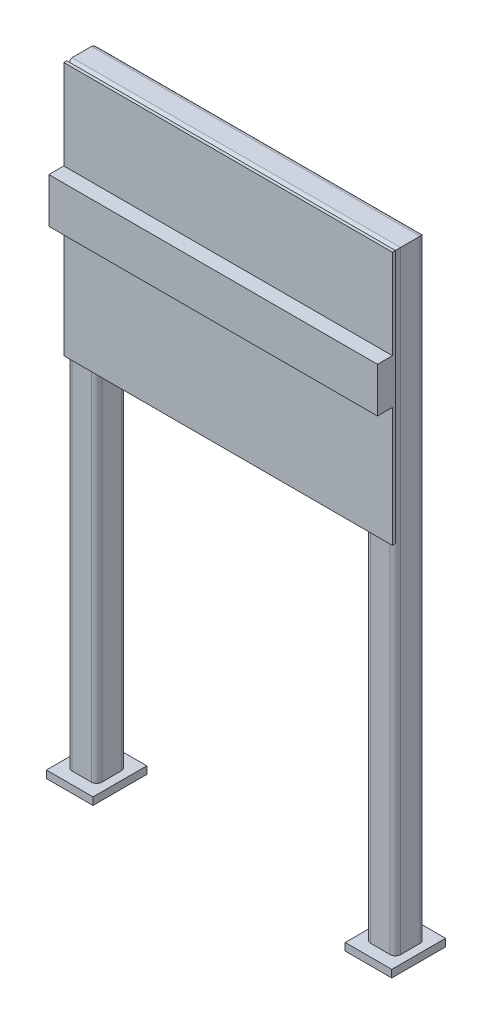
SolidWorks part; units mm, degrees
ref_plane "Front Plane" through (0, 0, 0) normal (0, 0, 1) x (1, 0, 0)
ref_plane "Top Plane" through (0, 0, 0) normal (0, 1, 0) x (1, 0, 0)
ref_plane "Right Plane" through (0, 0, 0) normal (1, 0, 0) x (0, 0, -1)
sketch "草图1" plane through (0, 0, 0) normal (0, 0, 1) x (1, 0, 0)
  line L0 (0, 0) -> (0, 116.4338) construction
  line L1 (-100, 0) -> (-100, 400)
  line L2 (100, 0) -> (100, 400)
  line L3 (-100, 250) -> (100, 250)
  line L4 (-100, 400) -> (100, 400)
  line L5 (-100, 330) -> (100, 330)
  dimension "D1" = 200
  dimension "D2" = 400
  dimension "D3" = 250
  dimension "D4" = 80
other "GB/6728-1986 square hollow section 020 X 20 X 1.75(1)"
ref_plane "Plane1" through (-100, 0, 0) normal (0, 1, 0) x (-1, 0, 0)
sketch "Sketch1" plane through (-100, 0, 0) normal (0, 1, 0) x (-1, 0, 0)
  line L0 (-6.5, -8.25) -> (6.5, -8.25)
  line L1 (-8.25, -6.5) -> (-8.25, 6.5)
  line L2 (6.5, 8.25) -> (-6.5, 8.25)
  line L3 (8.25, 6.5) -> (8.25, -6.5)
  line L4 (-6.5, -10) -> (6.5, -10)
  line L5 (-10, -6.5) -> (-10, 6.5)
  line L6 (6.5, 10) -> (-6.5, 10)
  line L7 (10, 6.5) -> (10, -6.5)
  arc A0 (10, 6.5) -> (6.5, 10) centre (6.5, 6.5) ccw
  arc A1 (6.5, -10) -> (10, -6.5) centre (6.5, -6.5) ccw
  arc A2 (-10, -6.5) -> (-6.5, -10) centre (-6.5, -6.5) ccw
  arc A3 (-6.5, 10) -> (-10, 6.5) centre (-6.5, 6.5) ccw
  arc A4 (-6.5, 8.25) -> (-8.25, 6.5) centre (-6.5, 6.5) ccw
  arc A5 (8.25, 6.5) -> (6.5, 8.25) centre (6.5, 6.5) ccw
  arc A6 (6.5, -8.25) -> (8.25, -6.5) centre (6.5, -6.5) ccw
  arc A7 (-8.25, -6.5) -> (-6.5, -8.25) centre (-6.5, -6.5) ccw
  point P0 (-10, 0)
  point P1 (10, 0)
  point P2 (0, 10)
  point P3 (0, -10)
  point P4 (0, 0)
  point P5 (-10, -10)
  point P6 (10, -10)
  point P7 (10, 10)
  point P8 (-10, 10)
  point P33 (0, 0)
  dimension "D1" = 3.5
  dimension "Thickness" = 1.75
  dimension "V_leg" = 20
sketch "Sketch2" plane through (0, 0, 0) normal (0, -1, 0) x (1, 0, 0)
  line L0 (0, 0) -> (0, 61.2443) construction
  line L1 (-110, 0) -> (-90, 0) construction
  line L2 (-110, -6.5) -> (-110, 6.5) construction
  line L3 (-90, -6.5) -> (-90, 6.5) construction
  line L4 (115.587, 18.0185) -> (84.413, -18.0185) construction
  line L5 (-115.587, -18.0185) -> (-84.413, -18.0185)
  line L6 (-115.587, -18.0185) -> (-115.587, 18.0185)
  line L7 (-115.587, 18.0185) -> (-84.413, 18.0185)
  line L8 (-84.413, -18.0185) -> (-84.413, 18.0185)
  line L9 (-115.587, -18.0185) -> (-84.413, 18.0185) construction
  line L10 (-115.587, 18.0185) -> (-84.413, -18.0185) construction
  line L11 (115.587, -18.0185) -> (84.413, 18.0185) construction
  line L12 (110, 0) -> (90, 0) construction
  line L13 (84.413, -18.0185) -> (84.413, 18.0185)
  line L14 (115.587, 18.0185) -> (84.413, 18.0185)
  line L15 (115.587, -18.0185) -> (115.587, 18.0185)
  line L16 (115.587, -18.0185) -> (84.413, -18.0185)
  point P9 (-100, 0)
  point P20 (100, 0)
extrude "Boss-Extrude1" add sketch "Sketch2" along normal blind 5
sketch "Sketch3" plane through (0, 0, 10) normal (0, 0, 1) x (1, 0, 0)
  line L0 (110, 0) -> (110, 410) construction
  line L1 (-110, 410) -> (110, 410)
  line L2 (-110, 410) -> (-110, 240)
  line L3 (-110, 240) -> (110, 240)
  line L4 (110, 410) -> (110, 240)
  line L5 (90, 240) -> (-90, 240) construction
extrude "Boss-Extrude2" add sketch "Sketch3" along normal blind 2
sketch "Sketch4" plane through (0, 0, 12) normal (0, 0, 1) x (1, 0, 0)
  line L0 (-110, 410) -> (-110, 240) construction
  line L1 (-110, 350) -> (110, 350)
  line L2 (-110, 350) -> (-110, 320)
  line L3 (-110, 320) -> (110, 320)
  line L4 (110, 350) -> (110, 320)
  line L5 (110, 240) -> (110, 410) construction
  line L6 (110, 410) -> (-110, 410) construction
  dimension "D1" = 60
  dimension "D2" = 30
extrude "Boss-Extrude3" add sketch "Sketch4" along normal blind 10
